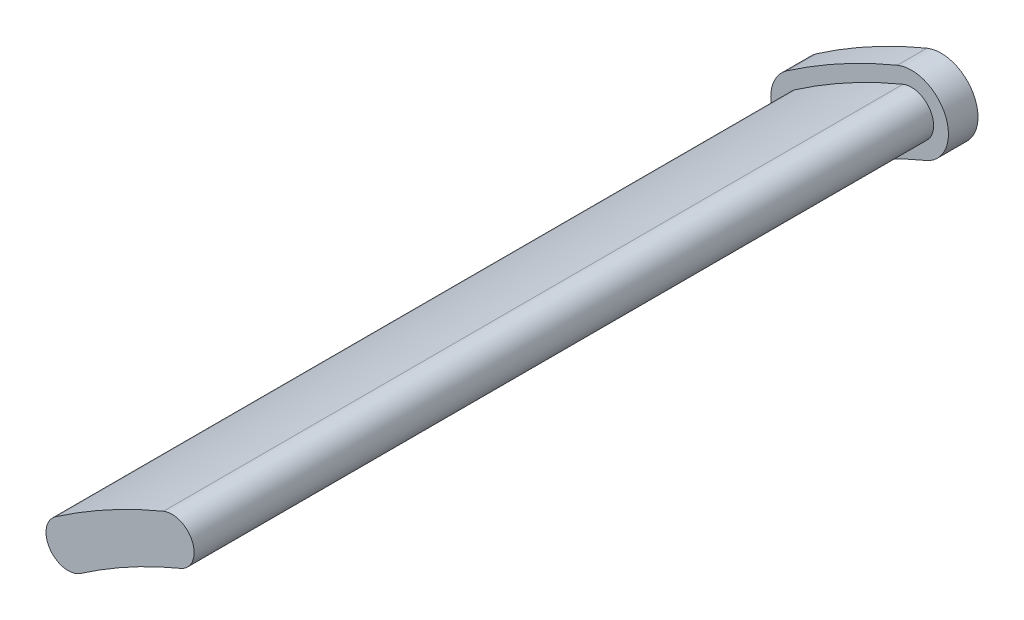
from build123d import *

# Parameters (mm, degrees)
BOSS_EXTRUDE1_DEPTH      = 20
BOSS_EXTRUDE1_DEPTH_BACK = 230
BOSS_EXTRUDE2_DEPTH      = 10


with BuildPart() as part:
    # Sketch1 → Boss-Extrude1 (new, two sides: drawn at the far end of the back side and taken through both)
    with BuildSketch(Plane.XY.offset(-BOSS_EXTRUDE1_DEPTH_BACK)):
        with BuildLine():
            ThreePointArc((-367.185078684, 365.188666312), (-385.937282785, 356.235559249), (-403.644999576, 345.361735137))
            ThreePointArc((-403.644999576, 345.361735137), (-405.565426886, 334.930438049), (-395.134129798, 333.010010739))
            ThreePointArc((-395.134129798, 333.010010739), (-378.77130289, 343.057974791), (-361.443316822, 351.33109904))
            ThreePointArc((-361.443316822, 351.33109904), (-357.385414117, 361.130763607), (-367.185078684, 365.188666312))
        make_face()
    extrude(amount=BOSS_EXTRUDE1_DEPTH + BOSS_EXTRUDE1_DEPTH_BACK)

    # Sketch2 → Boss-Extrude2 (add)
    with BuildSketch(Plane(origin=(0, 0, -230), x_dir=(-1, 0, 0), z_dir=(0, 0, -1))):
        with BuildLine():
            ThreePointArc((406.481956169, 349.478976603), (388.32594275, 360.628087401), (369.098999305, 369.807855403))
            ThreePointArc((369.098999305, 369.807855403), (352.766225026, 363.044684228), (359.529396201, 346.711909949))
            ThreePointArc((359.529396201, 346.711909949), (376.382642925, 338.665446638), (392.297173205, 328.892769272))
            ThreePointArc((392.297173205, 328.892769272), (409.682668352, 332.093481456), (406.481956169, 349.478976603))
        make_face()
    extrude(amount=BOSS_EXTRUDE2_DEPTH)


solid = part.part
